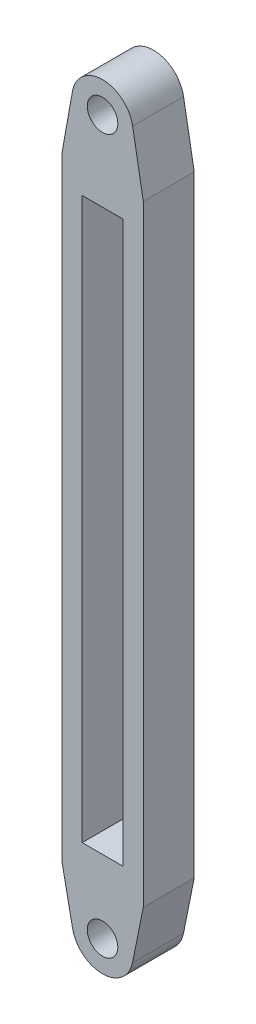
SolidWorks part; units mm, degrees
ref_plane "Front Plane" through (0, 0, 0) normal (0, 0, 1) x (1, 0, 0)
ref_plane "Top Plane" through (0, 0, 0) normal (0, 1, 0) x (1, 0, 0)
ref_plane "Right Plane" through (0, 0, 0) normal (1, 0, 0) x (0, 0, -1)
sketch "Sketch1" plane through (0, 0, 0) normal (0, 0, 1) x (1, 0, 0)
  line L0 (2.1187, -10.4911) -> (0, 0)
  line L2 (0, 0) -> (0, 120)
  line L4 (16, 0) -> (16, 120)
  line L5 (4, 115) -> (12, 115)
  line L6 (4, 115) -> (4, 5)
  line L7 (4, 5) -> (12, 5)
  line L8 (12, 115) -> (12, 5)
  line L9 (16, 0) -> (13.8813, -10.4911)
  line L10 (0, 120) -> (2.093, 131.749)
  line L11 (16, 120) -> (13.907, 131.749)
  line L12 (8, 130.6967) -> (8, -9.3033) construction
  circle A0 centre (8, 130.6967) radius 3
  circle A1 centre (8, -9.3033) radius 3
  arc A2 (13.907, 131.749) -> (2.093, 131.749) centre (8, 130.6967) ccw
  arc A3 (2.1187, -10.4911) -> (13.8813, -10.4911) centre (8, -9.3033) ccw
  dimension "D7" = 6
  dimension "D8" = 6
  dimension "D9" = 12
  dimension "D10" = 12
  dimension "D11" = 140
  dimension "D12" = 5
  dimension "D1" = 8
  dimension "D2" = 4
  dimension "D3" = 16
  dimension "D4" = 120
  dimension "D5" = 8
  dimension "D6" = 110
extrude "Boss-Extrude1" add sketch "Sketch1" along normal blind 10
